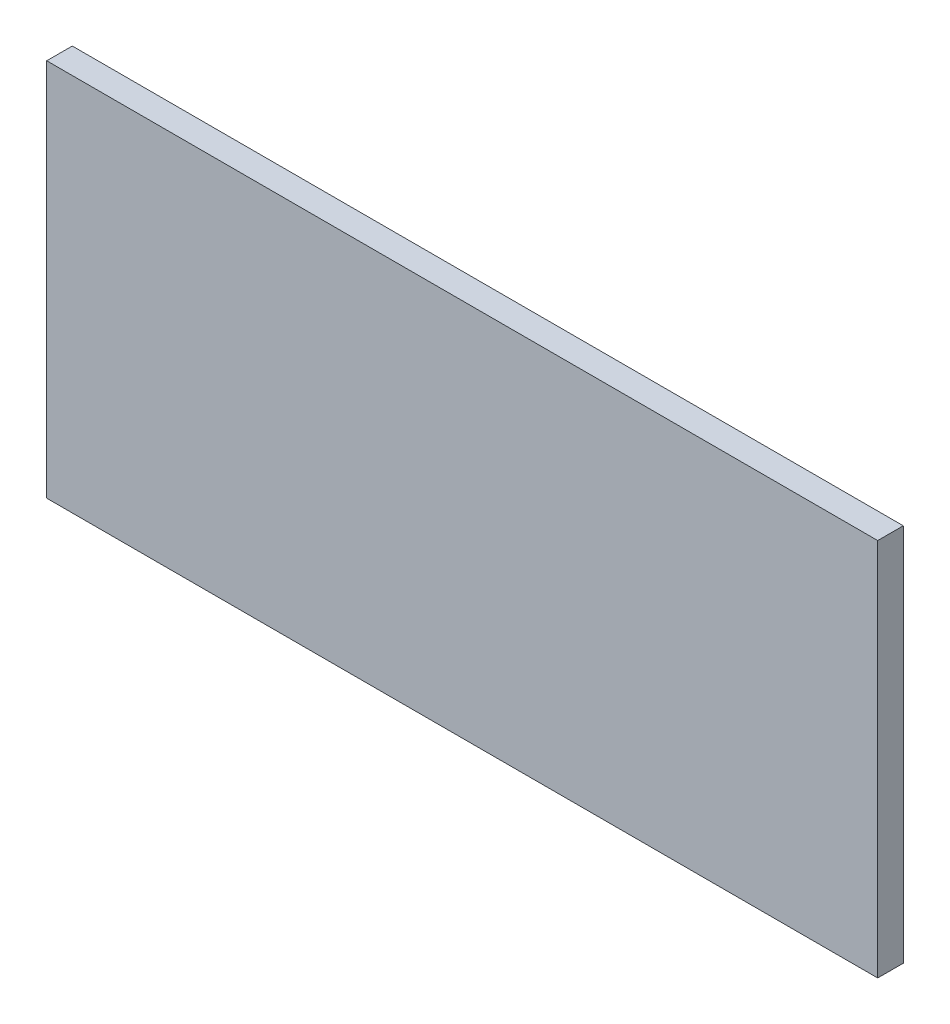
from build123d import *

# Parameters (mm, degrees)
SKETCH1_W      = 390
SKETCH1_H      = 177.8
EXTRUDE1_DEPTH = 6


with BuildPart() as part:
    # Sketch1 → Extrude1 (new, symmetric)
    with BuildSketch(Plane.XY):
        Rectangle(SKETCH1_W, SKETCH1_H)
    extrude(amount=EXTRUDE1_DEPTH, both=True)


solid = part.part
